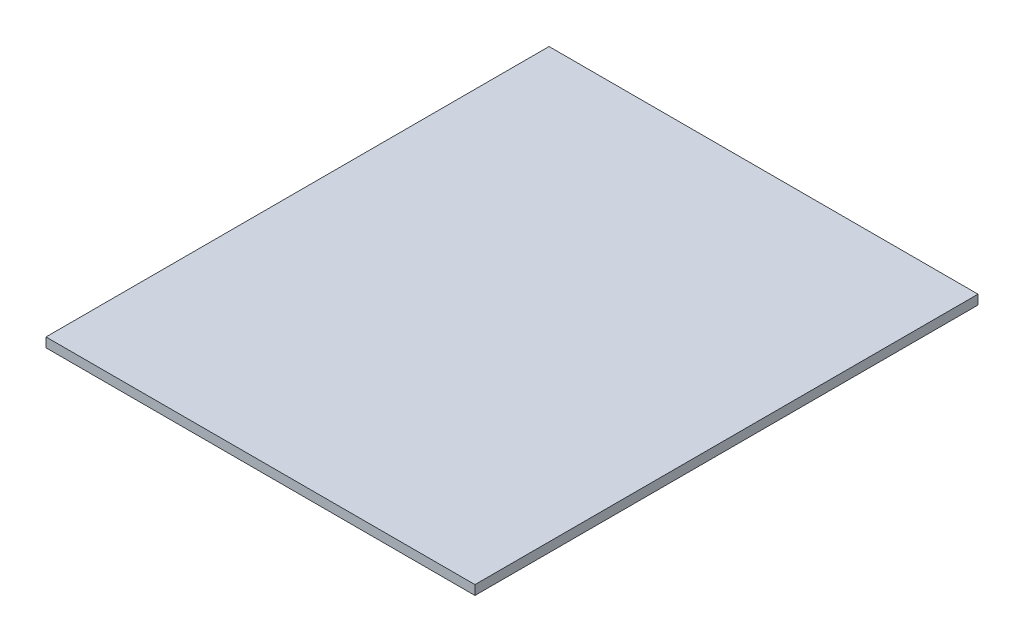
SolidWorks part; units mm, degrees
ref_plane "Front Plane" through (0, 0, 0) normal (0, 0, 1) x (1, 0, 0)
ref_plane "Top Plane" through (0, 0, 0) normal (0, 1, 0) x (1, 0, 0)
ref_plane "Right Plane" through (0, 0, 0) normal (1, 0, 0) x (0, 0, -1)
other "Configuration Table"
sketch "Sketch1" plane through (0, 0, 0) normal (0, 1, 0) x (1, 0, 0)
  line L1 (0, 0) -> (463.2, 0)
  line L2 (0, 0) -> (0, 543.2)
  line L3 (0, 543.2) -> (463.2, 543.2)
  line L4 (463.2, 0) -> (463.2, 543.2)
  dimension "D1" = 543.2
  dimension "D2" = 463.2
extrude "Boss-Extrude1" add sketch "Sketch1" along normal blind 10.2
